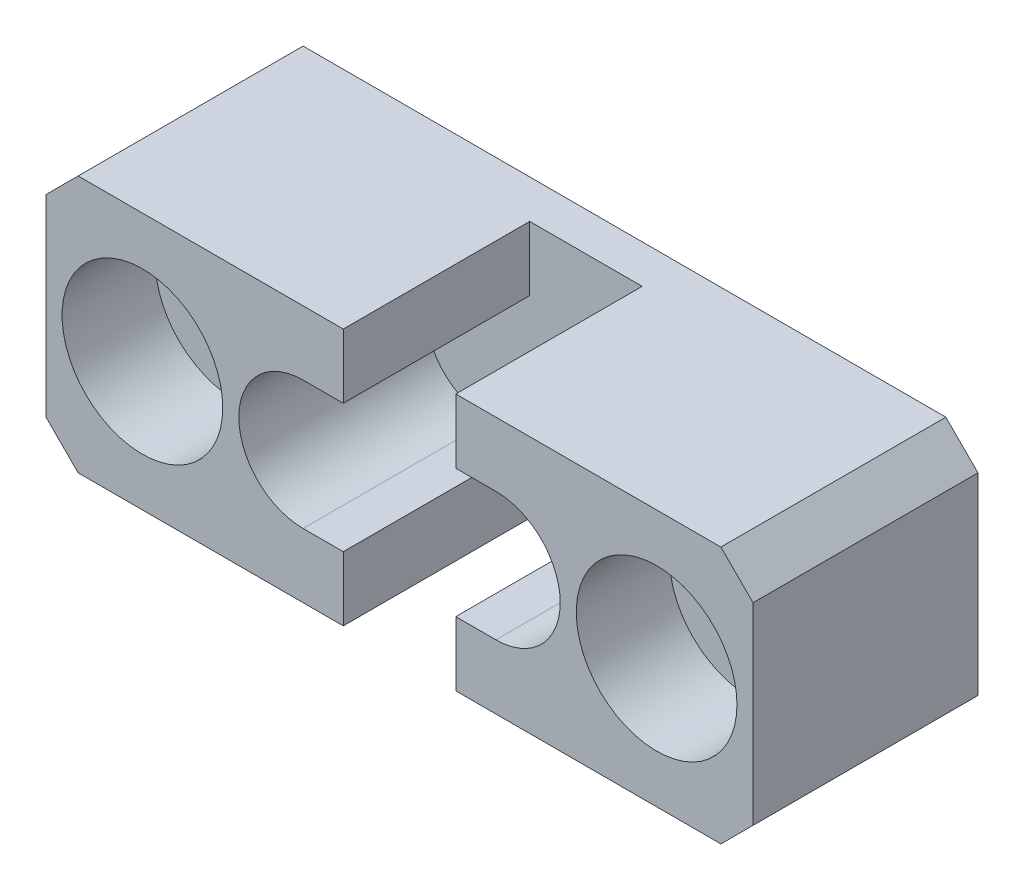
SolidWorks part; units mm, degrees
ref_plane "Front Plane" through (0, 0, 0) normal (0, 0, 1) x (1, 0, 0)
ref_plane "Top Plane" through (0, 0, 0) normal (0, 1, 0) x (1, 0, 0)
ref_plane "Right Plane" through (0, 0, 0) normal (1, 0, 0) x (0, 0, -1)
sketch "Sketch1" plane through (0, 0, 0) normal (0, 0, 1) x (1, 0, 0)
  line L1 (-11, -4) -> (11, -4)
  line L2 (-11, -4) -> (-11, 4)
  line L3 (-11, 4) -> (11, 4)
  line L4 (11, -4) -> (11, 4)
  line L5 (-11, -4) -> (11, 4) construction
  line L6 (-11, 4) -> (11, -4) construction
  point P0 (0, 0)
  dimension "D1" = 22
  dimension "D2" = 8
extrude "Boss-Extrude1" add sketch "Sketch1" along normal blind 7
sketch "Sketch3" plane through (0, 0, 7) normal (0, 0, 1) x (1, 0, 0)
  line L0 (0, 5.8471) -> (0, -7.7354) construction
  line L1 (-3, 2) -> (-1.75, 2)
  line L2 (-3, -2) -> (-1.75, -2)
  line L3 (-1.75, 4) -> (-1.75, 2)
  line L4 (11, 4) -> (-11, 4) construction
  line L5 (1.75, 4) -> (1.75, 2)
  line L6 (-1.75, 4) -> (1.75, 4)
  line L7 (-1.75, -4) -> (1.75, -4)
  line L8 (-11, -4) -> (11, -4) construction
  line L9 (1.75, -2) -> (1.75, -4)
  line L10 (-1.75, -2) -> (-1.75, -4)
  line L11 (1.75, -2) -> (3, -2)
  line L12 (1.75, 2) -> (3, 2)
  arc A0 (-3, 2) -> (-3, -2) centre (-3, 0) ccw
  arc A1 (3, 2) -> (3, -2) centre (3, 0) cw
  dimension "D3" = 4
  dimension "D1" = 6
  dimension "D2" = 3.5
extrude "Cut-Extrude1" cut sketch "Sketch3" against normal blind 5.8
chamfer "Chamfer1" distance 1 angle 45 4 edges at (11, -4, 3.5) (11, 4, 3.5) (-11, -4, 3.5) (-11, 4, 3.5)
hole_wizard "Hole size per socket head cap screw type 1" positions "Sketch5" profile "Sketch4" counterbore size "M2.5" standard "Gb" end condition through all
sketch "Sketch5" plane through (0, 0, 7) normal (0, 0, 1) x (1, 0, 0)
  line L0 (0, 0) -> (0, 8.8594) construction
  line L2 (0, 0) -> (15.7678, 0) construction
  point P0 (-8, 0)
  point P2 (8, 0)
  dimension "D1" = 16
sketch "Sketch4" plane through (-8, 0, 7) normal (1, 0, 0) x (0, -1, 0)
  line L0 (0, 0) -> (0, 7)
  line L1 (0, 7) -> (1.45, 7)
  line L3 (1.45, 7) -> (1.45, 2.9)
  line L4 (1.45, 2.9) -> (2.5, 2.9)
  line L5 (2.5, 2.9) -> (2.5, 0)
  line L7 (2.5, 0) -> (0, 0)
  line L11 (0, -6.35) -> (0, 107.95) construction
  dimension "通孔孔直径" = 2.9
  dimension "通孔孔深度" = 7
  dimension "柱形沉头孔直径" = 5
  dimension "柱形沉头孔深度" = 2.9
